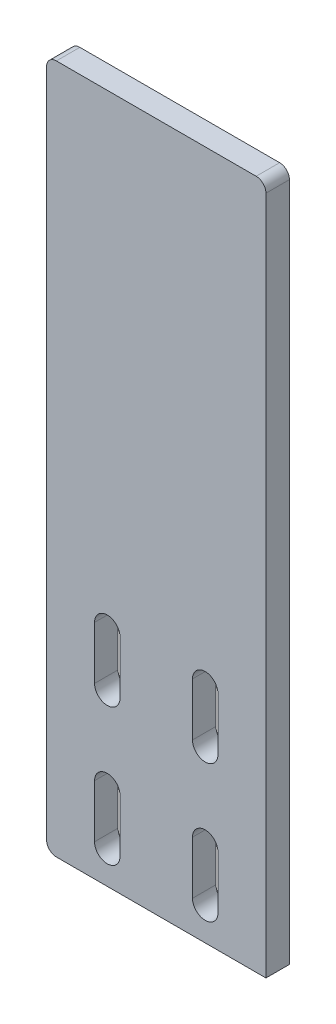
SolidWorks part; units mm, degrees
material "1023 碳钢板 (SS)"
ref_plane "Front Plane" through (0, 0, 0) normal (0, 0, 1) x (1, 0, 0)
ref_plane "Top Plane" through (0, 0, 0) normal (0, 1, 0) x (1, 0, 0)
ref_plane "Right Plane" through (0, 0, 0) normal (1, 0, 0) x (0, 0, -1)
sketch "Sketch1" plane through (0, 0, 0) normal (0, 0, 1) x (1, 0, 0)
  line L0 (-25, -62.5) -> (-25, -89.5) construction
  line L1 (-56, 176) -> (56, 176)
  line L2 (-56, 176) -> (-56, -176)
  line L3 (-56, -176) -> (56, -176)
  line L4 (56, 176) -> (56, -176)
  line L5 (-56, 176) -> (56, -176) construction
  line L6 (-56, -176) -> (56, 176) construction
  line L7 (-18.5, -62.5) -> (-18.5, -89.5)
  line L8 (-31.5, -62.5) -> (-31.5, -89.5)
  line L9 (25, -62.5) -> (25, -89.5) construction
  line L10 (31.5, -62.5) -> (31.5, -89.5)
  line L11 (18.5, -62.5) -> (18.5, -89.5)
  line L12 (-31.5, -132.5) -> (-31.5, -159.5)
  line L13 (-18.5, -132.5) -> (-18.5, -159.5)
  line L14 (18.5, -132.5) -> (18.5, -159.5)
  line L15 (31.5, -132.5) -> (31.5, -159.5)
  line L16 (-25, -132.5) -> (-25, -159.5) construction
  line L17 (25, -132.5) -> (25, -159.5) construction
  arc A0 (-18.5, -62.5) -> (-31.5, -62.5) centre (-25, -62.5) ccw
  arc A1 (-31.5, -89.5) -> (-18.5, -89.5) centre (-25, -89.5) ccw
  arc A2 (31.5, -62.5) -> (18.5, -62.5) centre (25, -62.5) ccw
  arc A3 (18.5, -89.5) -> (31.5, -89.5) centre (25, -89.5) ccw
  arc A4 (-18.5, -132.5) -> (-31.5, -132.5) centre (-25, -132.5) ccw
  arc A5 (-31.5, -159.5) -> (-18.5, -159.5) centre (-25, -159.5) ccw
  arc A6 (31.5, -132.5) -> (18.5, -132.5) centre (25, -132.5) ccw
  arc A7 (18.5, -159.5) -> (31.5, -159.5) centre (25, -159.5) ccw
  point P0 (0, 0)
  point P8 (-25, -76)
  point P13 (25, -76)
  point P24 (-25, -146)
  point P29 (25, -146)
  dimension "D5" = 6.5
  dimension "D6" = 6.5
  dimension "D7" = 50
  dimension "D8" = 31
  dimension "D1" = 112
  dimension "D2" = 352
  dimension "D3" = 27
  dimension "D4" = 27
  dimension "D10" = 43
  dimension "D11" = 16.5
  dimension "D9" = 2
extrude "Boss-Extrude1" add sketch "Sketch1" along normal blind 12
fillet "Fillet1" radius 5 3 edges at (-56, -176, 6) (56, 176, 6) (-56, 176, 6)
